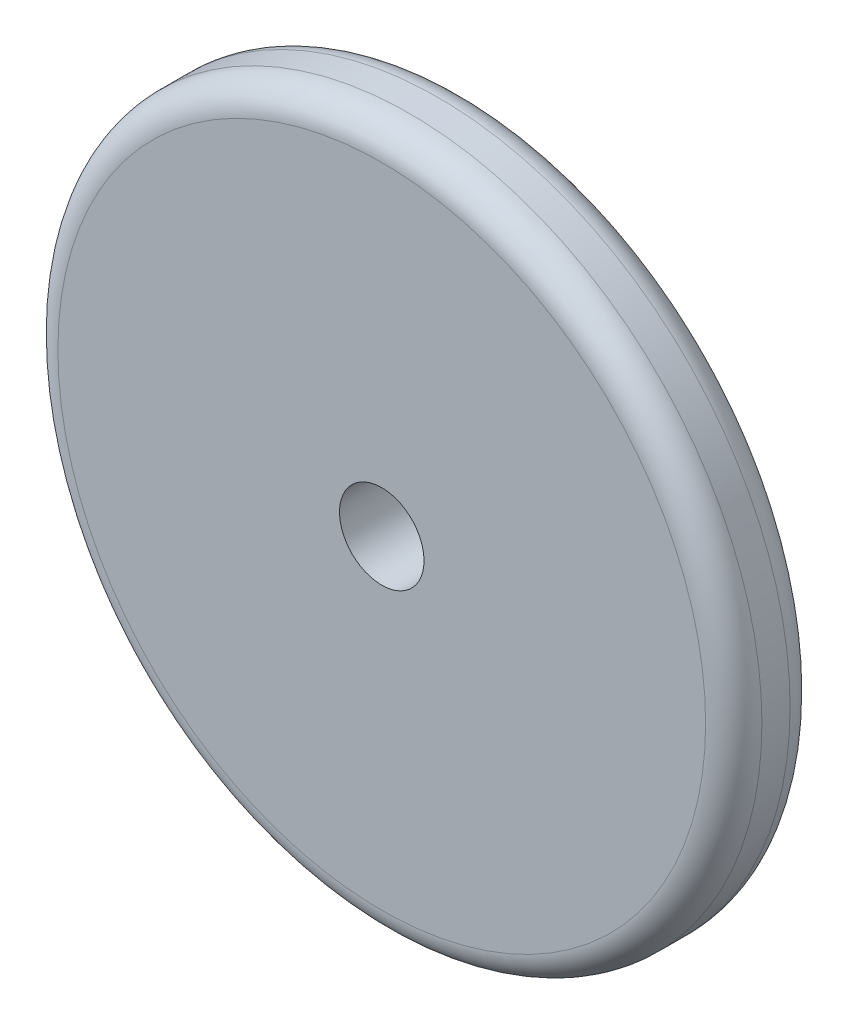
SolidWorks part; units mm, degrees
ref_plane "Front Plane" through (0, 0, 0) normal (0, 0, 1) x (1, 0, 0)
ref_plane "Top Plane" through (0, 0, 0) normal (0, 1, 0) x (1, 0, 0)
ref_plane "Right Plane" through (0, 0, 0) normal (1, 0, 0) x (0, 0, -1)
sketch "Model" plane through (0, 0, 0) normal (0, 0, 1) x (1, 0, 0)
  circle A0 centre (-26.873, -17.8946) radius 25
  circle A1 centre (-26.873, -17.8946) radius 3
  dimension "D1" = 6
  dimension "D2" = 50
extrude "Boss-Extrude1" add sketch "Model" along normal blind 6
fillet "Fillet1" radius 2 2 edges at (-1.873, -17.8946, 6) (-1.873, -17.8946, 0)
